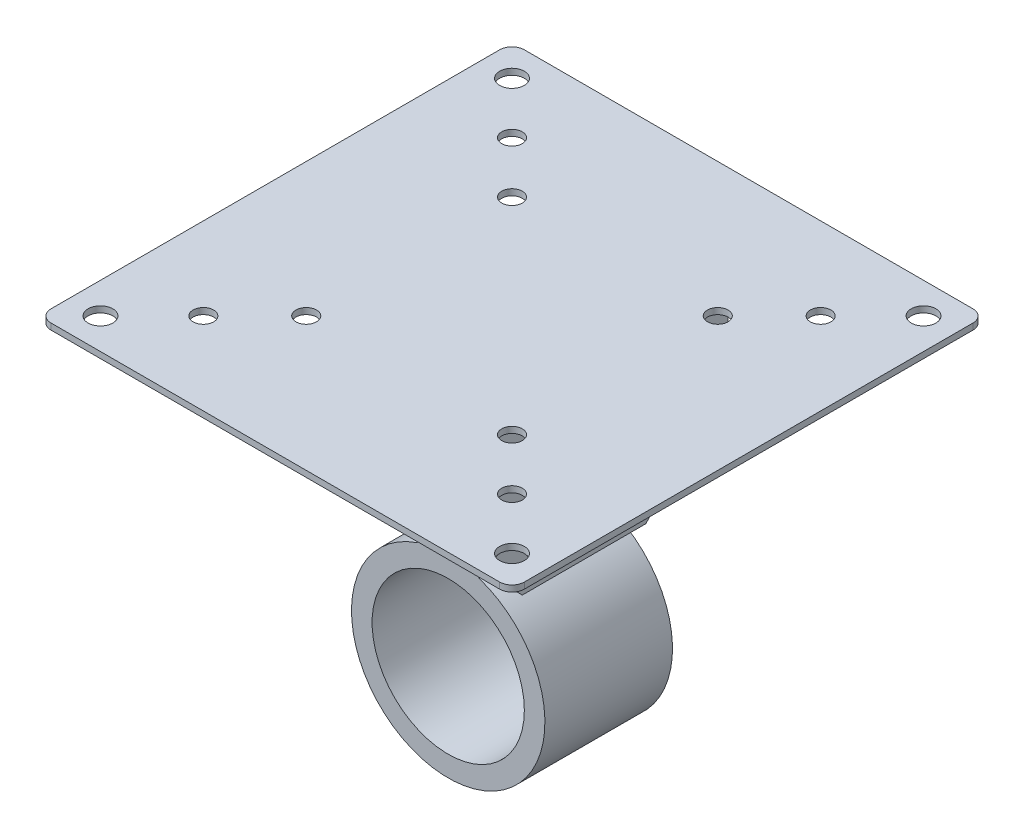
SolidWorks part; units mm, degrees
material "6061"
ref_plane "前视基准面" through (0, 0, 0) normal (0, 0, 1) x (1, 0, 0)
ref_plane "上视基准面" through (0, 0, 0) normal (0, 1, 0) x (1, 0, 0)
ref_plane "右视基准面" through (0, 0, 0) normal (1, 0, 0) x (0, 0, -1)
sketch "草图1" plane through (0, 0, 0) normal (0, 1, 0) x (1, 0, 0)
  line L1 (57.5, -57.5) -> (-57.5, -57.5)
  line L2 (57.5, -57.5) -> (57.5, 57.5)
  line L3 (57.5, 57.5) -> (-57.5, 57.5)
  line L4 (-57.5, -57.5) -> (-57.5, 57.5)
  line L5 (57.5, -57.5) -> (-57.5, 57.5) construction
  line L6 (57.5, 57.5) -> (-57.5, -57.5) construction
  point P0 (0, 0)
  dimension "D1" = 115
  dimension "D2" = 115
extrude "凸台-拉伸1" add sketch "草图1" along normal mid plane 1.5
sketch "草图2" plane through (0, 0.75, 0) normal (0, 1, 0) x (1, 0, 0)
  line L1 (-25, -25) -> (25, -25) construction
  line L2 (-25, -25) -> (-25, 25) construction
  line L3 (-25, 25) -> (25, 25) construction
  line L4 (25, -25) -> (25, 25) construction
  line L5 (-25, -25) -> (25, 25) construction
  line L6 (-25, 25) -> (25, -25) construction
  circle A0 centre (-25, 25) radius 2.5
  circle A1 centre (25, 25) radius 2.5
  circle A2 centre (25, -25) radius 2.5
  circle A3 centre (-25, -25) radius 2.5
  point P0 (0, 0)
  dimension "D3" = 5
  dimension "D1" = 50
  dimension "D2" = 50
extrude "切除-拉伸1" cut sketch "草图2" against normal through all
sketch "草图3" plane through (0, 0.75, 0) normal (0, 1, 0) x (1, 0, 0)
  line L1 (-37.5, 37.5) -> (37.5, 37.5) construction
  line L2 (-37.5, 37.5) -> (-37.5, -37.5) construction
  line L3 (-37.5, -37.5) -> (37.5, -37.5) construction
  line L4 (37.5, 37.5) -> (37.5, -37.5) construction
  line L5 (-37.5, 37.5) -> (37.5, -37.5) construction
  line L6 (-37.5, -37.5) -> (37.5, 37.5) construction
  circle A0 centre (-37.5, 37.5) radius 2.5
  circle A1 centre (-37.5, -37.5) radius 2.5
  circle A2 centre (37.5, -37.5) radius 2.5
  circle A3 centre (37.5, 37.5) radius 2.5
  point P0 (0, 0)
  dimension "D3" = 5
  dimension "D1" = 75
  dimension "D2" = 75
extrude "切除-拉伸2" cut sketch "草图3" against normal through all
sketch "草图4" plane through (0, 0.75, 0) normal (0, 1, 0) x (1, 0, 0)
  line L1 (-50, 50) -> (50, 50) construction
  line L2 (-50, 50) -> (-50, -50) construction
  line L3 (-50, -50) -> (50, -50) construction
  line L4 (50, 50) -> (50, -50) construction
  line L5 (-50, 50) -> (50, -50) construction
  line L6 (-50, -50) -> (50, 50) construction
  circle A0 centre (-50, 50) radius 3
  circle A1 centre (50, 50) radius 3
  circle A2 centre (-50, -50) radius 3
  circle A3 centre (50, -50) radius 3
  point P0 (0, 0)
  dimension "D3" = 6
  dimension "D1" = 100
  dimension "D2" = 100
extrude "切除-拉伸3" cut sketch "草图4" against normal through all
fillet "圆角1" radius 3 4 edges at (-57.5, 0, 57.5) (57.5, 0, 57.5) (57.5, 0, -57.5) (-57.5, 0, -57.5)
sketch "草图5" plane through (0, -0.75, 0) normal (0, -1, 0) x (1, 0, 0)
  line L1 (17.5, -35) -> (-17.5, -35)
  line L2 (17.5, -35) -> (17.5, 35)
  line L3 (17.5, 35) -> (-17.5, 35)
  line L4 (-17.5, -35) -> (-17.5, 35)
  line L5 (17.5, -35) -> (-17.5, 35) construction
  line L6 (17.5, 35) -> (-17.5, -35) construction
  point P0 (0, 0)
  dimension "D1" = 70
  dimension "D2" = 35
extrude "凸台-拉伸2" add sketch "草图5" along normal blind 41
chamfer "倒角1" distance 20 angle 45 2 edges at (0, -41.75, 35) (0, -41.75, -35)
sketch "草图6" plane through (0, 0, 0) normal (0, 0, 1) x (1, 0, 0)
  line L0 (0, 0) -> (0, -90.3647) construction
  line L1 (-17.5, -41.75) -> (17.5, -41.75) construction
  line L2 (7.5, -41.75) -> (7.5, -42.9789)
  line L4 (-7.5, -42.9789) -> (-7.5, -41.75)
  line L5 (-7.5, -41.75) -> (7.5, -41.75)
  arc A0 (-7.5, -42.9789) -> (7.5, -42.9789) centre (0, -65.25) ccw
  circle A1 centre (0, -65.25) radius 18.5
  point P7 (0, -65.25)
  point P11 (22.4732, -58.3793)
  point P16 (18.5, -65.25)
  dimension "D1" = 47
  dimension "D2" = 37
  dimension "D3" = 15
extrude "凸台-拉伸3" add sketch "草图6" along normal mid plane 31
